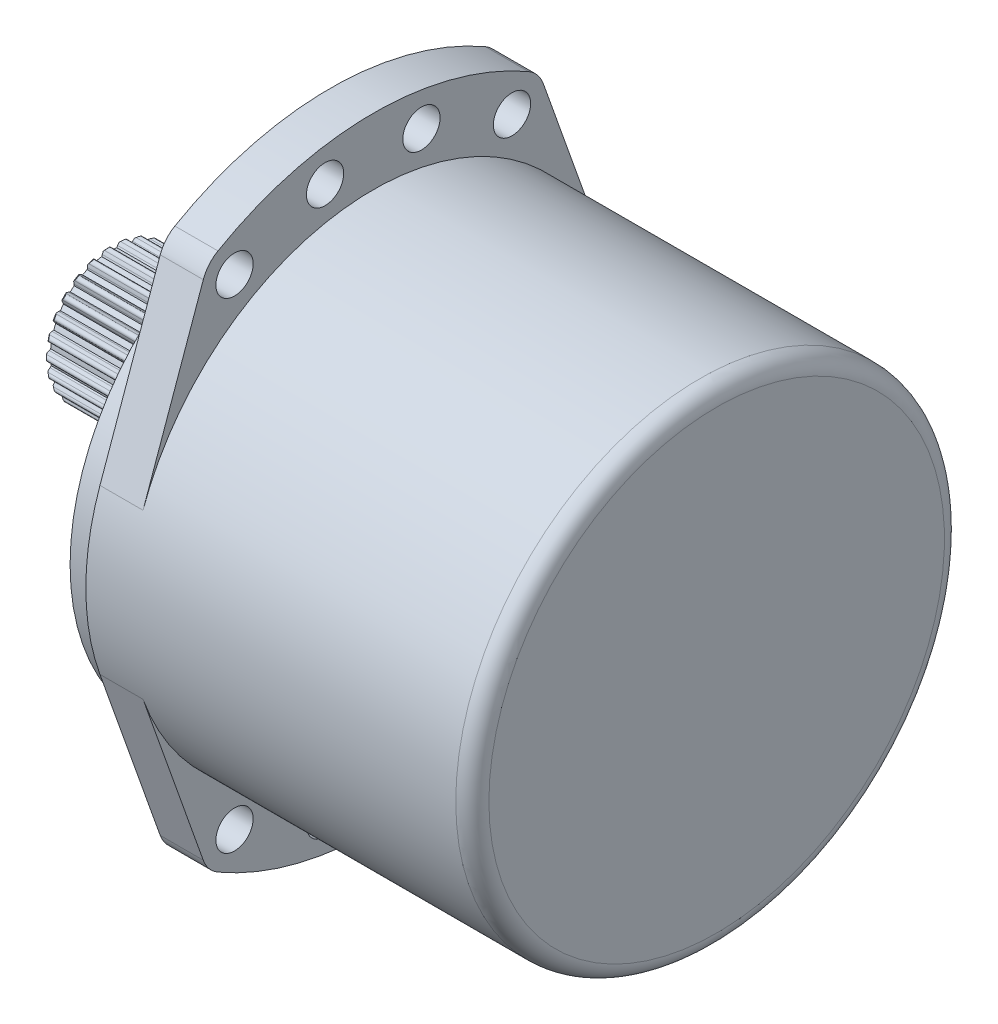
from build123d import *
from build123d.topology import SkipClean

# Parameters (mm, degrees)
CUT_EXTRUDE1_REACH  = 355.187
SKETCH2_R           = 11.25
BOSS_EXTRUDE1_REACH = 438.885


with BuildPart() as part:
    # Sketch1 → Revolve1 (revolve)
    with BuildSketch(Plane.XY, mode=Mode.PRIVATE) as revolve1_sk:
        with BuildLine():
            Line((-207.3, 187.5), (-207.3, 147.5))
            Line((-207.3, 147.5), (-10, 147.5))
            ThreePointArc((-10, 147.5), (-2.928932, 144.571068), (0, 137.5))
            Line((0, 137.5), (0, 0))
            Line((0, 0), (-366, 0))
            Line((-366, 0), (-366, 35))
            Line((-366, 35), (-283.8, 35))
            Line((-283.8, 35), (-283.8, 43))
            Line((-283.8, 43), (-280.8, 43))
            Line((-280.8, 43), (-280.8, 88))
            Line((-280.8, 88), (-250.3, 88))
            Line((-250.3, 88), (-250.3, 140))
            Line((-250.3, 140), (-233.3, 140))
            Line((-233.3, 140), (-233.3, 187.5))
            Line((-233.3, 187.5), (-207.3, 187.5))
        make_face()
    revolve(revolve1_sk.sketch.rotate(Axis((-112.339332, 0, 0), (1, 0, 0)), 90), axis=Axis((-112.339332, 0, 0), (1, 0, 0)))

    # Sketch2 → Cut-Extrude1 (cut, up to next)
    with BuildSketch(Plane.ZY.offset(233.3), mode=Mode.PRIVATE) as cut_extrude1_sk1:
        with Locations((-83.75, 145.059255)):
            Circle(SKETCH2_R)
    cut_extrude1_tool1 = extrude(cut_extrude1_sk1.sketch, amount=-CUT_EXTRUDE1_REACH, mode=Mode.PRIVATE) & part.part
    # Sketch2 → Cut-Extrude1 (cut, up to next)
    with BuildSketch(Plane.ZY.offset(233.3), mode=Mode.PRIVATE) as cut_extrude1_sk2:
        with Locations((-29.08607, 164.955299)):
            Circle(SKETCH2_R)
    cut_extrude1_tool2 = extrude(cut_extrude1_sk2.sketch, amount=-CUT_EXTRUDE1_REACH, mode=Mode.PRIVATE) & part.part
    # Sketch2 → Cut-Extrude1 (cut, up to next)
    with BuildSketch(Plane.ZY.offset(233.3), mode=Mode.PRIVATE) as cut_extrude1_sk3:
        with Locations((29.08607, 164.955299)):
            Circle(SKETCH2_R)
    cut_extrude1_tool3 = extrude(cut_extrude1_sk3.sketch, amount=-CUT_EXTRUDE1_REACH, mode=Mode.PRIVATE) & part.part
    # Sketch2 → Cut-Extrude1 (cut, up to next)
    with BuildSketch(Plane.ZY.offset(233.3), mode=Mode.PRIVATE) as cut_extrude1_sk4:
        with Locations((83.75, 145.059255)):
            Circle(SKETCH2_R)
    cut_extrude1_tool4 = extrude(cut_extrude1_sk4.sketch, amount=-CUT_EXTRUDE1_REACH, mode=Mode.PRIVATE) & part.part
    # Sketch2 → Cut-Extrude1 (cut, up to next)
    with BuildSketch(Plane.ZY.offset(233.3), mode=Mode.PRIVATE) as cut_extrude1_sk5:
        with Locations((83.75, -145.059255)):
            Circle(SKETCH2_R)
    cut_extrude1_tool5 = extrude(cut_extrude1_sk5.sketch, amount=-CUT_EXTRUDE1_REACH, mode=Mode.PRIVATE) & part.part
    # Sketch2 → Cut-Extrude1 (cut, up to next)
    with BuildSketch(Plane.ZY.offset(233.3), mode=Mode.PRIVATE) as cut_extrude1_sk6:
        with Locations((29.08607, -164.955299)):
            Circle(SKETCH2_R)
    cut_extrude1_tool6 = extrude(cut_extrude1_sk6.sketch, amount=-CUT_EXTRUDE1_REACH, mode=Mode.PRIVATE) & part.part
    # Sketch2 → Cut-Extrude1 (cut, up to next)
    with BuildSketch(Plane.ZY.offset(233.3), mode=Mode.PRIVATE) as cut_extrude1_sk7:
        with Locations((-29.08607, -164.955299)):
            Circle(SKETCH2_R)
    cut_extrude1_tool7 = extrude(cut_extrude1_sk7.sketch, amount=-CUT_EXTRUDE1_REACH, mode=Mode.PRIVATE) & part.part
    # Sketch2 → Cut-Extrude1 (cut, up to next)
    with BuildSketch(Plane.ZY.offset(233.3), mode=Mode.PRIVATE) as cut_extrude1_sk8:
        with Locations((-83.75, -145.059255)):
            Circle(SKETCH2_R)
    cut_extrude1_tool8 = extrude(cut_extrude1_sk8.sketch, amount=-CUT_EXTRUDE1_REACH, mode=Mode.PRIVATE) & part.part
    # Sketch2 → Cut-Extrude1 (cut, up to next)
    with BuildSketch(Plane.ZY.offset(233.3), mode=Mode.PRIVATE) as cut_extrude1_sk9:
        with BuildLine():
            Line((-102.594709, 151.75828), (-138.97973, 49.405311))
            ThreePointArc((-138.97973, 49.405311), (-147.5, 0), (-138.97973, -49.405311))
            Line((-138.97973, -49.405311), (-102.594709, -151.75828))
            ThreePointArc((-102.594709, -151.75828), (-99.119069, -157.857369), (-93.75, -162.379763))
            ThreePointArc((-93.75, -162.379763), (-187.5, 0), (-93.75, 162.379763))
            ThreePointArc((-93.75, 162.379763), (-99.119069, 157.857369), (-102.594709, 151.75828))
        make_face()
    cut_extrude1_tool9 = extrude(cut_extrude1_sk9.sketch, amount=-CUT_EXTRUDE1_REACH, mode=Mode.PRIVATE) & part.part
    # Sketch2 → Cut-Extrude1 (cut, up to next)
    with BuildSketch(Plane.ZY.offset(233.3), mode=Mode.PRIVATE) as cut_extrude1_sk10:
        with BuildLine():
            Line((102.594709, 151.75828), (138.97973, 49.405311))
            ThreePointArc((138.97973, 49.405311), (147.5, 0), (138.97973, -49.405311))
            Line((138.97973, -49.405311), (102.594709, -151.75828))
            ThreePointArc((102.594709, -151.75828), (99.119069, -157.857369), (93.75, -162.379763))
            ThreePointArc((93.75, -162.379763), (187.5, 0), (93.75, 162.379763))
            ThreePointArc((93.75, 162.379763), (99.119069, 157.857369), (102.594709, 151.75828))
        make_face()
    cut_extrude1_tool10 = extrude(cut_extrude1_sk10.sketch, amount=-CUT_EXTRUDE1_REACH, mode=Mode.PRIVATE) & part.part
    add(cut_extrude1_tool1.solids().sort_by_distance((-233.3, 145.059255, -83.75))[0], mode=Mode.SUBTRACT)
    add(cut_extrude1_tool2.solids().sort_by_distance((-233.3, 164.955299, -29.08607))[0], mode=Mode.SUBTRACT)
    add(cut_extrude1_tool3.solids().sort_by_distance((-233.3, 164.955299, 29.08607))[0], mode=Mode.SUBTRACT)
    add(cut_extrude1_tool4.solids().sort_by_distance((-233.3, 145.059255, 83.75))[0], mode=Mode.SUBTRACT)
    add(cut_extrude1_tool5.solids().sort_by_distance((-233.3, -145.059255, 83.75))[0], mode=Mode.SUBTRACT)
    add(cut_extrude1_tool6.solids().sort_by_distance((-233.3, -164.955299, 29.08607))[0], mode=Mode.SUBTRACT)
    add(cut_extrude1_tool7.solids().sort_by_distance((-233.3, -164.955299, -29.08607))[0], mode=Mode.SUBTRACT)
    add(cut_extrude1_tool8.solids().sort_by_distance((-233.3, -145.059255, -83.75))[0], mode=Mode.SUBTRACT)
    add(cut_extrude1_tool9.solids().sort_by_distance((-233.3, 0, -150.135342))[0], mode=Mode.SUBTRACT)
    add(cut_extrude1_tool10.solids().sort_by_distance((-233.3, 0, 150.135342))[0], mode=Mode.SUBTRACT)

    # Sketch5 → Boss-Extrude1 (add, up to next)
    with BuildSketch(Plane.ZY.offset(366), mode=Mode.PRIVATE) as boss_extrude1_sk1:
        with BuildLine():
            ThreePointArc((37.201834, -11.195805), (38.706319, -9.938094), (37.993836, -8.111161))
            ThreePointArc((37.993836, -8.111161), (37.23616, -7.381947), (36.440112, -6.694827))
            ThreePointArc((36.440112, -6.694827), (36.042393, -6.380193), (35.635453, -6.077578))
            ThreePointArc((35.635453, -6.077578), (35.864946, -4.530796), (36.027332, -2.975537))
            ThreePointArc((36.027332, -2.975537), (36.496745, -2.783632), (36.960215, -2.577791))
            ThreePointArc((36.960215, -2.577791), (37.902133, -2.110227), (38.817353, -1.592349))
            ThreePointArc((38.817353, -1.592349), (39.961792, 0), (38.817353, 1.592349))
            ThreePointArc((38.817353, 1.592349), (37.902133, 2.110227), (36.960215, 2.577791))
            ThreePointArc((36.960215, 2.577791), (36.496745, 2.783632), (36.027332, 2.975537))
            ThreePointArc((36.027332, 2.975537), (35.864946, 4.530796), (35.635453, 6.077578))
            ThreePointArc((35.635453, 6.077578), (36.042393, 6.380193), (36.440112, 6.694827))
            ThreePointArc((36.440112, 6.694827), (37.23616, 7.381947), (37.993836, 8.111161))
            ThreePointArc((37.993836, 8.111161), (38.706319, 9.938094), (37.201834, 11.195805))
            ThreePointArc((37.201834, 11.195805), (36.186576, 11.469807), (35.157971, 11.688436))
            ThreePointArc((35.157971, 11.688436), (34.657871, 11.77255), (34.155482, 11.841688))
            ThreePointArc((34.155482, 11.841688), (33.61142, 13.307703), (33.004468, 14.748817))
            ThreePointArc((33.004468, 14.748817), (33.323366, 15.143126), (33.630343, 15.546784))
            ThreePointArc((33.630343, 15.546784), (34.230502, 16.410286), (34.783026, 17.305017))
            ThreePointArc((34.783026, 17.305017), (35.018785, 19.25174), (33.248786, 20.095788))
            ThreePointArc((33.248786, 20.095788), (32.197283, 20.108698), (31.146623, 20.064655))
            ThreePointArc((31.146623, 20.064655), (30.641316, 20.021756), (30.137516, 19.963783))
            ThreePointArc((30.137516, 19.963783), (29.245964, 21.248437), (28.29969, 22.493333))
            ThreePointArc((28.29969, 22.493333), (28.510509, 22.954561), (28.707456, 23.42188))
            ThreePointArc((28.707456, 23.42188), (29.074016, 24.407506), (29.38667, 25.411535))
            ThreePointArc((29.38667, 25.411535), (29.130893, 27.355729), (27.206595, 27.733079))
            ThreePointArc((27.206595, 27.733079), (26.184916, 27.484085), (25.178218, 27.180137))
            ThreePointArc((25.178218, 27.180137), (24.699455, 27.012921), (24.2259, 26.831479))
            ThreePointArc((24.2259, 26.831479), (23.042877, 27.854054), (21.816739, 28.82451))
            ThreePointArc((21.816739, 28.82451), (21.906232, 29.323676), (21.980774, 29.825292))
            ThreePointArc((21.980774, 29.825292), (22.090702, 30.871113), (22.143842, 31.921352))
            ThreePointArc((22.143842, 31.921352), (21.412599, 33.740857), (19.454914, 33.627798))
            ThreePointArc((19.454914, 33.627798), (18.527255, 33.132546), (17.627773, 32.587791))
            ThreePointArc((17.627773, 32.587791), (17.205636, 32.306765), (16.792081, 32.013255))
            ThreePointArc((16.792081, 32.013255), (15.391921, 32.709498), (13.962962, 33.344538))
            ThreePointArc((13.962962, 33.344538), (13.925505, 33.850277), (13.872959, 34.354672))
            ThreePointArc((13.872959, 34.354672), (13.719348, 35.394975), (13.509635, 36.425434))
            ThreePointArc((13.509635, 36.425434), (12.348873, 38.005923), (10.480808, 37.40956))
            ThreePointArc((10.480808, 37.40956), (9.705458, 36.699167), (8.96971, 35.947834))
            ThreePointArc((8.96971, 35.947834), (8.630723, 35.570656), (8.303154, 35.183521))
            ThreePointArc((8.303154, 35.183521), (6.773835, 35.509684), (5.23184, 35.769405))
            ThreePointArc((5.23184, 35.769405), (5.069788, 36.249941), (4.893455, 36.725422))
            ThreePointArc((4.893455, 36.725422), (4.485957, 37.69484), (4.026568, 38.640772))
            ThreePointArc((4.026568, 38.640772), (2.509222, 39.882936), (0.848155, 38.840741))
            ThreePointArc((0.848155, 38.840741), (0.273832, 37.959844), (-0.251953, 37.049143))
            ThreePointArc((-0.251953, 37.049143), (-0.486489, 36.599512), (-0.70749, 36.143076))
            ThreePointArc((-0.70749, 36.143076), (-2.269877, 36.078666), (-3.828017, 35.946749))
            ThreePointArc((-3.828017, 35.946749), (-4.104482, 36.371887), (-4.393523, 36.788578))
            ThreePointArc((-4.393523, 36.788578), (-5.029303, 37.626199), (-5.709503, 38.428168))
            ThreePointArc((-5.709503, 38.428168), (-7.488093, 39.253959), (-8.83779, 37.831415))
            ThreePointArc((-8.83779, 37.831415), (-9.175, 36.835365), (-9.457785, 35.822518))
            ThreePointArc((-9.457785, 35.822518), (-9.573134, 35.328686), (-9.673681, 34.831629))
            ThreePointArc((-9.673681, 34.831629), (-11.170964, 34.380693), (-12.647346, 33.865427))
            ThreePointArc((-12.647346, 33.865427), (-13.020853, 34.208454), (-13.404439, 34.540172))
            ThreePointArc((-13.404439, 34.540172), (-14.228553, 35.193366), (-15.086825, 35.800981))
            ThreePointArc((-15.086825, 35.800981), (-17.014903, 36.15851), (-17.968425, 34.445002))
            ThreePointArc((-17.968425, 34.445002), (-18.047334, 33.396385), (-18.069349, 32.345033))
            ThreePointArc((-18.069349, 32.345033), (-18.058263, 31.838029), (-18.032038, 31.331583))
            ThreePointArc((-18.032038, 31.331583), (-19.370139, 30.522455), (-20.671995, 29.656215))
            ThreePointArc((-20.671995, 29.656215), (-21.119076, 29.895579), (-21.573106, 30.121481))
            ThreePointArc((-21.573106, 30.121481), (-22.533771, 30.549205), (-23.516187, 30.924286))
            ThreePointArc((-23.516187, 30.924286), (-25.472605, 30.79109), (-25.970038, 28.894284))
            ThreePointArc((-25.970038, 28.894284), (-25.785687, 27.858986), (-25.54555, 26.83519))
            ThreePointArc((-25.54555, 26.83519), (-25.408726, 26.346871), (-25.257377, 25.862858))
            ThreePointArc((-25.257377, 25.862858), (-26.352216, 24.746378), (-27.397748, 23.583595))
            ThreePointArc((-27.397748, 23.583595), (-27.890309, 23.704253), (-28.386255, 23.810146))
            ThreePointArc((-28.386255, 23.810146), (-29.42311, 23.985524), (-30.46794, 24.104505))
            ThreePointArc((-30.46794, 24.104505), (-32.329769, 23.488952), (-32.339858, 21.528031))
            ThreePointArc((-32.339858, 21.528031), (-31.90383, 20.571106), (-31.416629, 19.639193))
            ThreePointArc((-31.416629, 19.639193), (-31.162664, 19.200243), (-30.895701, 18.769075))
            ThreePointArc((-30.895701, 18.769075), (-31.678486, 17.415395), (-32.401998, 16.02913))
            ThreePointArc((-32.401998, 16.02913), (-32.909092, 16.023503), (-33.415791, 16.002732))
            ThreePointArc((-33.415791, 16.002732), (-34.463686, 15.914745), (-35.50528, 15.770149))
            ThreePointArc((-35.50528, 15.770149), (-37.155534, 14.710917), (-36.677645, 12.809093))
            ThreePointArc((-36.677645, 12.809093), (-36.017339, 11.990667), (-35.313687, 11.209194))
            ThreePointArc((-35.313687, 11.209194), (-34.958538, 10.847193), (-34.592735, 10.495961))
            ThreePointArc((-34.592735, 10.495961), (-35.014281, 8.990139), (-35.370312, 7.467496))
            ThreePointArc((-35.370312, 7.467496), (-35.860075, 7.335937), (-36.34569, 7.189807))
            ThreePointArc((-36.34569, 7.189807), (-37.338782, 6.843984), (-38.311693, 6.444897))
            ThreePointArc((-38.311693, 6.444897), (-39.646681, 5.008541), (-38.710841, 3.285312))
            ThreePointArc((-38.710841, 3.285312), (-37.867745, 2.65681), (-36.991856, 2.074879))
            ThreePointArc((-36.991856, 2.074879), (-36.557838, 1.812573), (-36.11618, 1.563348))
            ThreePointArc((-36.11618, 1.563348), (-36.15, 0), (-36.11618, -1.563348))
            ThreePointArc((-36.11618, -1.563348), (-36.557838, -1.812573), (-36.991856, -2.074879))
            ThreePointArc((-36.991856, -2.074879), (-37.867745, -2.65681), (-38.710841, -3.285312))
            ThreePointArc((-38.710841, -3.285312), (-39.646681, -5.008541), (-38.311693, -6.444897))
            ThreePointArc((-38.311693, -6.444897), (-37.338782, -6.843984), (-36.34569, -7.189807))
            ThreePointArc((-36.34569, -7.189807), (-35.860075, -7.335937), (-35.370312, -7.467496))
            ThreePointArc((-35.370312, -7.467496), (-35.014281, -8.990139), (-34.592735, -10.495961))
            ThreePointArc((-34.592735, -10.495961), (-34.958538, -10.847193), (-35.313687, -11.209194))
            ThreePointArc((-35.313687, -11.209194), (-36.017339, -11.990667), (-36.677645, -12.809093))
            ThreePointArc((-36.677645, -12.809093), (-37.155534, -14.710917), (-35.50528, -15.770149))
            ThreePointArc((-35.50528, -15.770149), (-34.463686, -15.914745), (-33.415791, -16.002732))
            ThreePointArc((-33.415791, -16.002732), (-32.909092, -16.023503), (-32.401998, -16.02913))
            ThreePointArc((-32.401998, -16.02913), (-31.678486, -17.415395), (-30.895701, -18.769075))
            ThreePointArc((-30.895701, -18.769075), (-31.162664, -19.200243), (-31.416629, -19.639193))
            ThreePointArc((-31.416629, -19.639193), (-31.90383, -20.571106), (-32.339858, -21.528031))
            ThreePointArc((-32.339858, -21.528031), (-32.329769, -23.488952), (-30.46794, -24.104505))
            ThreePointArc((-30.46794, -24.104505), (-29.42311, -23.985524), (-28.386255, -23.810146))
            ThreePointArc((-28.386255, -23.810146), (-27.890309, -23.704253), (-27.397748, -23.583595))
            ThreePointArc((-27.397748, -23.583595), (-26.352216, -24.746378), (-25.257377, -25.862858))
            ThreePointArc((-25.257377, -25.862858), (-25.408726, -26.346871), (-25.54555, -26.83519))
            ThreePointArc((-25.54555, -26.83519), (-25.785687, -27.858986), (-25.970038, -28.894284))
            ThreePointArc((-25.970038, -28.894284), (-25.472605, -30.79109), (-23.516187, -30.924286))
            ThreePointArc((-23.516187, -30.924286), (-22.533771, -30.549205), (-21.573106, -30.121481))
            ThreePointArc((-21.573106, -30.121481), (-21.119076, -29.895579), (-20.671995, -29.656215))
            ThreePointArc((-20.671995, -29.656215), (-19.370139, -30.522455), (-18.032038, -31.331583))
            ThreePointArc((-18.032038, -31.331583), (-18.058263, -31.838029), (-18.069349, -32.345033))
            ThreePointArc((-18.069349, -32.345033), (-18.047334, -33.396385), (-17.968425, -34.445002))
            ThreePointArc((-17.968425, -34.445002), (-17.014903, -36.15851), (-15.086825, -35.800981))
            ThreePointArc((-15.086825, -35.800981), (-14.228553, -35.193366), (-13.404439, -34.540172))
            ThreePointArc((-13.404439, -34.540172), (-13.020853, -34.208454), (-12.647346, -33.865427))
            ThreePointArc((-12.647346, -33.865427), (-11.170964, -34.380693), (-9.673681, -34.831629))
            ThreePointArc((-9.673681, -34.831629), (-9.573134, -35.328686), (-9.457785, -35.822518))
            ThreePointArc((-9.457785, -35.822518), (-9.175, -36.835365), (-8.83779, -37.831415))
            ThreePointArc((-8.83779, -37.831415), (-7.488093, -39.253959), (-5.709503, -38.428168))
            ThreePointArc((-5.709503, -38.428168), (-5.029303, -37.626199), (-4.393523, -36.788578))
            ThreePointArc((-4.393523, -36.788578), (-4.104482, -36.371887), (-3.828017, -35.946749))
            ThreePointArc((-3.828017, -35.946749), (-2.269877, -36.078666), (-0.70749, -36.143076))
            ThreePointArc((-0.70749, -36.143076), (-0.486489, -36.599512), (-0.251953, -37.049143))
            ThreePointArc((-0.251953, -37.049143), (0.273832, -37.959844), (0.848155, -38.840741))
            ThreePointArc((0.848155, -38.840741), (2.509222, -39.882936), (4.026568, -38.640772))
            ThreePointArc((4.026568, -38.640772), (4.485957, -37.69484), (4.893455, -36.725422))
            ThreePointArc((4.893455, -36.725422), (5.069788, -36.249941), (5.23184, -35.769405))
            ThreePointArc((5.23184, -35.769405), (6.773835, -35.509684), (8.303154, -35.183521))
            ThreePointArc((8.303154, -35.183521), (8.630723, -35.570656), (8.96971, -35.947834))
            ThreePointArc((8.96971, -35.947834), (9.705458, -36.699167), (10.480808, -37.40956))
            ThreePointArc((10.480808, -37.40956), (12.348873, -38.005923), (13.509635, -36.425434))
            ThreePointArc((13.509635, -36.425434), (13.719348, -35.394975), (13.872959, -34.354672))
            ThreePointArc((13.872959, -34.354672), (13.925505, -33.850277), (13.962962, -33.344538))
            ThreePointArc((13.962962, -33.344538), (15.391921, -32.709498), (16.792081, -32.013255))
            ThreePointArc((16.792081, -32.013255), (17.205636, -32.306765), (17.627773, -32.587791))
            ThreePointArc((17.627773, -32.587791), (18.527255, -33.132546), (19.454914, -33.627798))
            ThreePointArc((19.454914, -33.627798), (21.412599, -33.740857), (22.143842, -31.921352))
            ThreePointArc((22.143842, -31.921352), (22.090702, -30.871113), (21.980774, -29.825292))
            ThreePointArc((21.980774, -29.825292), (21.906232, -29.323676), (21.816739, -28.82451))
            ThreePointArc((21.816739, -28.82451), (23.042877, -27.854054), (24.2259, -26.831479))
            ThreePointArc((24.2259, -26.831479), (24.699455, -27.012921), (25.178218, -27.180137))
            ThreePointArc((25.178218, -27.180137), (26.184916, -27.484085), (27.206595, -27.733079))
            ThreePointArc((27.206595, -27.733079), (29.130893, -27.355729), (29.38667, -25.411535))
            ThreePointArc((29.38667, -25.411535), (29.074016, -24.407506), (28.707456, -23.42188))
            ThreePointArc((28.707456, -23.42188), (28.510509, -22.954561), (28.29969, -22.493333))
            ThreePointArc((28.29969, -22.493333), (29.245964, -21.248437), (30.137516, -19.963783))
            ThreePointArc((30.137516, -19.963783), (30.641316, -20.021756), (31.146623, -20.064655))
            ThreePointArc((31.146623, -20.064655), (32.197283, -20.108698), (33.248786, -20.095788))
            ThreePointArc((33.248786, -20.095788), (35.018785, -19.25174), (34.783026, -17.305017))
            ThreePointArc((34.783026, -17.305017), (34.230502, -16.410286), (33.630343, -15.546784))
            ThreePointArc((33.630343, -15.546784), (33.323366, -15.143126), (33.004468, -14.748817))
            ThreePointArc((33.004468, -14.748817), (33.61142, -13.307703), (34.155482, -11.841688))
            ThreePointArc((34.155482, -11.841688), (34.657871, -11.77255), (35.157971, -11.688436))
            ThreePointArc((35.157971, -11.688436), (36.186576, -11.469807), (37.201834, -11.195805))
        make_face()
    boss_extrude1_tool1 = extrude(boss_extrude1_sk1.sketch, amount=-BOSS_EXTRUDE1_REACH, mode=Mode.PRIVATE) - part.part
    add(boss_extrude1_tool1.solids().sort_by_distance((-366, 0, 0))[0])

    # Sketch7 → Cut-Revolve1 (revolve, cut)
    with SkipClean():  # the faces are left unmerged after this step: merging them gives an invalid solid
        with BuildSketch(Plane(origin=(0, 0, 0), x_dir=(1, 0, 0), z_dir=(0, 1, 0)), mode=Mode.PRIVATE) as cut_revolve1_sk:
            Polygon((-366.384036, 40.043964), (-364.384036, 40.043964), (-366.384036, 38.043964), align=None)
        revolve(cut_revolve1_sk.sketch.rotate(Axis((-112.339332, 0, 0), (-1, 0, 0)), 180), axis=Axis((-112.339332, 0, 0), (-1, 0, 0)), mode=Mode.SUBTRACT)


solid = part.part
